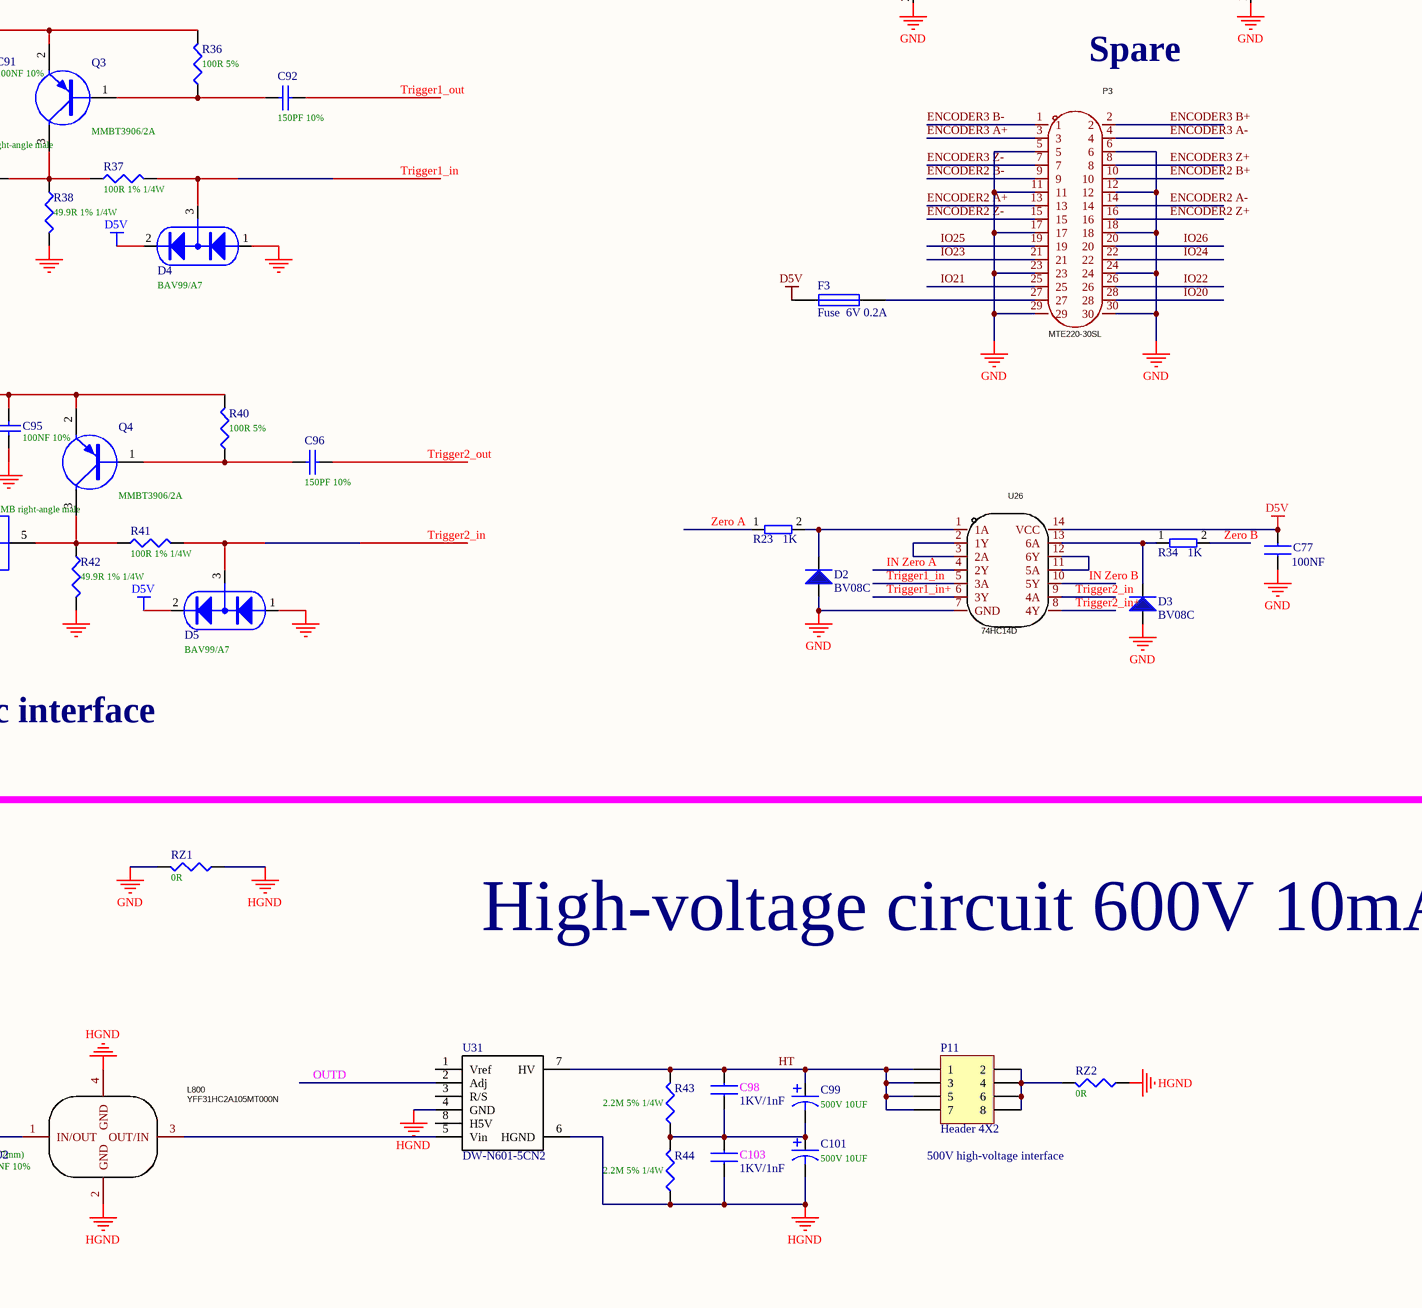
[diagram p0: MISC82191-3.SchDoc, bottom right]
# Altium project MISC82191-2.PrjPcb (part 2 of 4)

## Sheet MISC82191-3.SchDoc
size 965 x 596 mm

### Parts
C51  100NF 10%  [0805A]
C52  10pF/50V  [0603]
C53  10pF/50V  [0603]
C54  10pF/50V  [0603]
C55  10pF/50V  [0603]
C56  10pF/50V  [0603]
C57  10pF/50V  [0603]
C58  10pF/50V  [0603]
C59  10pF/50V  [0603]
C60  10pF/50V  [0603]
C61  100nF/50V  [0603]
C62  10pF/50V  [0603]
C63(NC)  10pF/50V  [0603]
C64  10pF/50V  [0603]
C65  10pF/50V  [0603]
C66  10pF/50V  [0603]
C67  10pF/50V  [0603]
C68（NC）  10pF/50V  [0603]
C69  100nF/50V  [0603]
C70  100nF/50V  [0603]
C71  100NF  [C0402]
C72  100NF  [C0402]
C73  100NF  [C0402]
C74  100NF  [C0402]
C75  100NF  [C0402]
C76  100NF  [C0402]
C77  100NF  [0603]
C78  100NF  [C0402]
C79  100NF  [C0402]
C80  100NF  [C0402]
C81  100NF  [C0402]
C82  100NF  [C0402]
C83  100NF  [C0402]
C85  100NF  [C0402]
C86  100NF  [C0402]
C87  100NF  [C0402]
C88  100NF  [C0402]
C89  100NF  [C0402]
C90  100NF  [C0402]
C91  100NF 10%  [0805R]
C92  150PF 10%  [0805R]
C95  100NF 10%  [0805R]
C96  150PF 10%  [0805R]
C97  10uF  25V 10%  [0805R]
C98  1KV/1nF  [3225[1210]]
C99  500V 10UF  [CAP-SMD_BD10.0-L10.3-W10.3-LS11.0-R-RD]
C100  220UF 25V (D6.3*7.7mm)  [CAP-SMD-6.3]
C101  500V 10UF  [CAP-SMD_BD10.0-L10.3-W10.3-LS11.0-R-RD]
C102  100NF 10%  [0805R]
C103  1KV/1nF  [3225[1210]]
C115  47uF 25V  [1206]
C116  47uF 25V  [1206]
C117  47uF 25V  [1206]
C501  100nF/50V  [0603]
C502  100nF/50V  [0603]
C704  10uF  25V 10%  [0805R]
C706  10uF  25V 10%  [0805R]
D2  BV08C  [SOD323]
D3  BV08C  [SOD323]
D4  BAV99/A7  [SOT-23]
D5  BAV99/A7  [SOT-23]
F1  Fuse  6V 0.2A  [0805]
F3  Fuse  6V 0.2A  [0805]
J1  0.8mm 2*50  [板对板座2*50]
J2  0.8mm 2*50  [板对板座2*50]
L11  600Ω-1.3A  [0805]
L12  600Ω-1.3A  [0805]
L13  600Ω-1.3A  [0805]
L14  600Ω-1.3A  [0805]
L15  600Ω-1.3A  [0805]
L16  600Ω-1.3A  [0805]
L17  600Ω-1.3A  [0805]
L18  600Ω-1.3A  [0805]
L19  600Ω-1.3A  [0805]
L20  XRCD54-4R7M(4.7uH 2A SMD,4.5x5.2mm)  [IND-SMD_L7.8-W7.0-A]
L80(NC)  600Ω-1.3A  [0805]
L104  YFF31HC2A105MT000N  [FILTER-SMD_4P-L3.2-W1.6-L_YFF31HC]
L105  YFF31HC2A105MT000N  [FILTER-SMD_4P-L3.2-W1.6-L_YFF31HC]
L106  YFF31HC2A105MT000N  [FILTER-SMD_4P-L3.2-W1.6-L_YFF31HC]
L800  YFF31HC2A105MT000N  [FILTER-SMD_4P-L3.2-W1.6-L_YFF31HC]
LED1  LED white body, red/green bicolour(Φ3/common anode) with 3mm single-hole square LED right-angle holder(7*6.4*7.4mm)  [DIP3B]
P2  Header 10  [2B-10]
P3  MTE220-30SL  [CONN-TH_MTE220-30SL]
P4  Header 20X2  [N0.8mm/40Pin-Plug]
P6  Header 20X2  [N0.8mm/40Pin-Plug]
P7  Header 7X2  [IDC-TH_14P-P2.54-V-R2-C7-S2.54]
P8  RF connector SMB-JWHD SMB right-angle male  [DIP-P]
P9  Header 20X2  [N0.8mm/40Pin-Plug]
P10  RF connector SMB-JWHD SMB right-angle male  [DIP-P]
P11  Header 4X2  [N0.8mm/8Pin-SOCKET]
P13  Header 20X2  [N0.8mm/40Pin-Plug]
P50  Analog output  [DIP-P]
P51  AD input  [DIP-P]
P52  gain  [DIP-P]
P53  (no value)  [DIP-P]
Q1  MMBT3904LT1(1AM)  [SOT23]
Q2  MMBT3904LT1(1AM)  [SOT23]
Q3  MMBT3906/2A  [SOT-23]
Q4  MMBT3906/2A  [SOT-23]
R19  100R 5%  [0603A]
R20  100R 5%  [0603A]
R23  1K  [0402]
R25  2K 5%  [0603A]
R26  2K 5%  [0603A]
R27  2K 5%  [0603A]
R28  2K 5%  [0603A]
R34  1K  [0402]
R35  100R 5%  [0805R]
R36  100R 5%  [0805R]
R37  100R 1% 1/4W  [AXIAL-0.45]
R38  49.9R 1% 1/4W  [AXIAL-0.5]
R39  100R 5%  [0805R]
R40  100R 5%  [0805R]
R41  100R 1% 1/4W  [AXIAL-0.45]
R42  49.9R 1% 1/4W  [AXIAL-0.5]
R43  2.2M 5% 1/4W  [AXIAL-0.5]
R44  2.2M 5% 1/4W  [AXIAL-0.5]
RJ1  HY911130A  [HY911130A]
RZ1  0R  [0805R]
RZ2  0R  [0805R]
U8  BV05C  [SOD-323]
U9  BV05C  [SOD-323]
U10  BV05C  [SOD-323]
U11  BV05C  [SOD-323]
U12  BV05C  [SOD-323]
U13  SMBJ33CA /33V  [DO-214AC(SMA)]
U14  BV05C  [SOD-323]
U15  BV05C  [SOD-323]
U16  BV05C  [SOD-323]
U17  AM26LV32EIPWR  [TSSOP-16_L5.0-W4.4-P0.65-LS6.4-BL]  (value not drawn)
U18  TXB0108RGYR  [QFN20]
U19  TXB0108RGYR  [QFN20]
U20  TXB0108RGYR  [QFN20]
U21  AM26LV32EIPWR  [TSSOP-16_L5.0-W4.4-P0.65-LS6.4-BL]  (value not drawn)
U22  AM26LV32EIPWR  [TSSOP-16_L5.0-W4.4-P0.65-LS6.4-BL]  (value not drawn)
U23  TXB0108RGYR  [QFN20]
U24  TXB0108RGYR  [QFN20]
U25  TXB0108RGYR  [QFN20]
U26  74HC14D  [SO-14]
U27  TXB0108RGYR  [QFN20]
U28  TXB0108RGYR  [QFN20]
U29  TXB0108RGYR  [QFN20]
U31  DW-N601-5CN2  [DW-N601-5CN2]
U501  74HC14D  [SO-14]
U707  74HC14D  [SO-14]

### Nets
3V3: C72.2 C74.2 C76.2 C79.2 C81.2 C83.2 C86.2 C90.2 LED1.2 P7.2 RJ1.11 RJ1.14 U18.2(VCCA) U18.10(OE) U19.2(VCCA) U19.10(OE) U20.2(VCCA) U20.10(OE) U23.2(VCCA) U23.10(OE) U24.2(VCCA) U24.10(OE) U25.2(VCCA) U25.10(OE) U27.2(VCCA) U27.10(OE) U29.2(VCCA) U29.10(OE)
13V: C115.1 C116.2 C117.2 J2.A1 J2.A2 J2.A3 J2.A4 J2.A5 J2.A6 J2.A7 J2.A8 J2.A9 J2.A10 J2.B1 J2.B2 J2.B3 J2.B4 J2.B5 J2.B6 J2.B7 J2.B8 J2.B9 J2.B10 L20.1 L106.3(OUT/IN)
-5.4V: L104.3(OUT/IN)
A6V: L105.3(OUT/IN)
A6V4: C706.2 L105.1(IN/OUT) P9.17 P9.18 P9.19 P9.20 P9.21 P9.22 P9.23 P9.24
D5V: C61.2 C69.2 C70.2 C71.1 C73.1 C75.1 C77.2 C78.1 C80.1 C82.1 C85.1 C87.1 C89.1 C501.2 C502.2 D4.2 D5.2 F1.2 F3.2 R35.2 R39.2 U17.4(G) U17.16(VCC) U18.19(VCCB) U19.19(VCCB) U20.19(VCCB) U21.4(G) U21.16(VCC) U22.4(G) U22.16(VCC) U23.19(VCCB) U24.19(VCCB) U25.19(VCCB) U26.14(VCC) U27.19(VCCB) U28.19(VCCB) U29.19(VCCB) U501.14(VCC) U707.14(VCC)
DGND: C54.2 C55.2 C59.2 C60.2 C61.1 C66.2 C67.1 C68（NC）.2 C69.1 C70.1 C71.2 C72.1 C73.2 C74.1 C75.2 C76.1 C77.1 C78.2 C79.1 C80.2 C81.1 C82.2 C83.1 C85.2 C86.1 C87.2 C88.1 C89.2 C90.1 C91.2 C95.2 C97.2 C115.2 C116.1 C117.1 C501.1 C502.1 C704.1 C706.1 D2.1 D3.1 D4.1 D5.1 J1.A2 J1.A5 J1.A8 J1.A11 J1.A14 J1.A17 J1.A20 J1.A23 J1.A25 J1.A28 J1.A31 J1.A34 J1.A37 J1.A40 J1.A42 J1.A45 J1.A48 J1.A50 J1.B2 J1.B5 J1.B8 J1.B11 J1.B14 J1.B17 J1.B20 J1.B23 J1.B25 J1.B28 J1.B31 J1.B34 J1.B37 J1.B40 J1.B42 J1.B45 J1.B48 J1.B50 J2.A11 J2.A12 J2.A13 J2.A14 J2.A15 J2.A16 J2.A17 J2.A18 J2.A19 J2.A20 J2.A23 J2.A26 J2.A29 J2.A32 J2.A35 J2.A38 J2.A41 J2.A44 J2.A47 J2.A50 J2.B11 J2.B12 J2.B13 J2.B14 J2.B15 J2.B16 J2.B17 J2.B18 J2.B19 J2.B20 J2.B21 J2.B22 J2.B23 J2.B24 J2.B26 J2.B29 J2.B32 J2.B35 J2.B38 J2.B41 J2.B44 J2.B47 J2.B50 L104.2(GND) L104.4(GND) L105.2(GND) L105.4(GND) L106.2(GND) L106.4(GND) P3.5 P3.6 P3.11 P3.12 P3.17 P3.18 P3.23 P3.24 P3.29 P3.30 P4.5 P4.6 P4.11 P4.12 P4.17 P4.18 P4.23 P4.24 P4.29 P4.30 P4.35 P4.36 P6.5 P6.6 P6.11 P6.12 P6.17 P6.18 P6.19 P6.23 P6.24 P6.29 P6.30 P6.35 P6.36 P7.3 P7.5 P7.7 P7.9 P7.11 P7.13 P8.1 P8.2 P8.3 P8.4 P9.11 P9.12 P9.13 P9.14 P9.15 P9.16 P9.25 P9.26 P9.27 P9.28 P9.29 P9.30 P10.1 P10.2 P10.3 P10.4 P13.9 P13.10 P13.11 P13.12 P13.17 P13.18 P13.23 P13.24 P13.25 P13.27 P13.29 P13.30 P13.31 P13.33 P13.35 P13.36 P13.37 P13.39 P50.1 P50.2 P50.3 P50.4 P51.1 P51.2 P51.3 P51.4 P52.1 P52.2 P52.3 P52.4 P53.1 P53.2 P53.3 P53.4 Q1.2(E) Q2.2(E) R27.1 R28.1 R38.1 R42.1 RZ1.2 U17.8(GND) U17.12(G#) U18.11(GND) U19.11(GND) U20.11(GND) U21.8(GND) U21.12(G#) U22.8(GND) U22.12(G#) U23.11(GND) U24.11(GND) U25.11(GND) U26.7(GND) U27.11(GND) U28.11(GND) U29.11(GND) U501.7(GND) U707.7(GND)  [also labelled GND]
HGND: C100.2 C101.2 C102.2 C103.2 L800.2(GND) L800.4(GND) R44.1 RZ1.1 RZ2.1 U31.4(GND) U31.6(HGND)
KGND: C51.2 C52.2 C53.2 C56.2 C57.2 C58.2 C62.1 C63(NC).1 C64.1 C65.1 P2.3 RJ1.10 RJ1.15(SH) RJ1.16(SH) U8.1 U9.1 U10.1 U11.1 U12.1 U13.2 U14.2 U15.2 U16.2
VCC1V8: C88.2 U28.2(VCCA) U28.10(OE)
1_A_N: C58.1 L14.2 P2.6 U12.2
1_A_P: C57.1 L13.2 P2.5 U11.2
1V8IO1: J1.A21
1V8IO2: J1.A22
1V8IO3: J1.A24
1V8IO4: J1.A27
1V8IO5: J1.A26
1V8IO6: J1.A29
1V8IO7: J1.A30
1V8IO8: J1.A32
1V8IO9: J1.A33
1V8IO10: J1.A35
1V8IO11: J1.A36
1V8IO12: J1.A38
1V8IO13: J1.A39
1V8IO14: J1.A41
1V8IO16: J1.A44
1V8IO17: J1.A46
1V8IO18: J1.A47
1V8IO19: P13.20 U28.1(A1)
1V8IO20: P13.22 U28.3(A2)
1V8IO21: P13.26 U28.4(A3)
1V8IO22: P13.28 U28.5(A4)
1V8IO23: P13.32 U28.6(A5)
1V8IO24: P13.34 U28.7(A6)
1V8IO25: P13.38 U28.8(A7)
1V8IO26: P13.40 U28.9(A8)
2_A_N: C65.2 L16.2 P2.8 U16.1
2_A_P: C52.1 L15.2 P2.7 U8.2
3_A_N: C63(NC).2 L18.2 L80(NC).2 P2.2 U14.1
3_A_P: C64.2 L17.2 P2.1 U15.1
3VIO23: J1.B19 U24.6(A5)
3VIO24: J1.B18 U24.5(A4)
3VIO25: J1.A18 U19.9(A8)
3VIO26: J1.B22 U24.8(A7)
3VIO27: J1.A4 U18.6(A5)
3VIO28: J1.B16 U19.8(A7)
3VIO29: J1.B15 U19.7(A6)
3VIO30: J1.B1 U18.5(A4)
3VIO31: J1.B3 U18.7(A6)
3VIO32: J1.A16 U19.6(A5)
3VIO33: J1.A15 U19.5(A4)
3VIO34: J1.B13 U19.3(A2)
3VIO40: J2.B27
3VIO41: J2.B28
3VIO42: J2.B30
3VIO43: J2.B25 U25.9(A8)
3VIO44: J2.B31 U25.4(A3)
3VIO45: J2.B33 U25.1(A1)
3VIO46: J2.B34 U20.8(A7)
3VIO47: J2.B36 U20.7(A6)
3VIO48: J2.B37 U20.6(A5)
3VIO49: J2.B39 U20.5(A4)
3VIO50: J2.B40 U20.4(A3)
3VIO51: J2.B42 U20.3(A2)
3VIO52: J2.B43 U20.1(A1)
3VIO53: J2.A27 U25.8(A7)
3VIO54: J2.A28 U25.7(A6)
3VIO55: J2.A30 U25.6(A5)
3VIO56: J2.A31 U25.5(A4)
3VIO57: J2.A33 U25.3(A2)
3VIO58: J2.A34 U20.9(A8)
3VIO60: J2.A37 U24.3(A2)
3VIO61: J2.A40 U19.4(A3)
3VIO62: J2.A39 U24.1(A1)
3VIO63: J2.A42
3VIO64: J2.A43
AK0: J2.A36 U24.4(A3)
AK1: P6.28 U27.12(B8)
AK2: P6.34 U27.13(B7)
AK3: P6.37 U27.17(B3)
AK4: P6.38 U27.14(B6)
AK5: P6.39 U27.16(B4)
AK6: P6.33 U27.18(B2)
AK7: P6.31 U27.20(B1)
AK8: P6.27 U29.12(B8)
AK9: P6.25 U29.13(B7)
AK10: P6.20 U29.17(B3)
AK11: U29.18(B2)
AK12: U29.15(B5)
AK13: P6.22 U29.16(B4)
AK16: U29.20(B1)
AS19: U24.13(B7)
AS20: P4.4 U18.15(B5)
AS23: P4.8 U18.16(B4)
AS24: P4.2 U18.14(B6)
AS27: P4.37 U19.18(B2)
AS28: P4.39 U19.17(B3)
Attn1: P4.33 U23.12(B8)
Attn2: P4.31 U23.13(B7)
Attn4: P4.27 U23.14(B6)
Attn8: P4.25 U23.15(B5)
Attn16: P4.21 U23.16(B4)
DAC Clk: J1.A7 P4.13
DAC Data: J1.B7 P4.15
DAC Strobe: J1.B6 P4.9
DATA_T: P6.40 U27.15(B5)
ENCODER2 A: U21.3(1Y) U501.13(6A)
ENCODER2 A+: P3.13 U21.2(1A)
ENCODER2 A-: P3.14 U21.1(1B)
ENCODER2 AA: U25.12(B8) U501.12(6Y)
ENCODER2 B: U21.5(2Y) U501.11(5A)
ENCODER2 B+: P3.10 U21.6(2A)
ENCODER2 B-: P3.9 U21.7(2B)
ENCODER2 BB: U25.13(B7) U501.10(5Y)
ENCODER2 Z: U21.11(3Y) U501.9(4A)
ENCODER2 Z+: P3.16 U21.10(3A)
ENCODER2 Z-: P3.15 U21.9(3B)
ENCODER2 ZZ: U25.14(B6) U501.8(4Y)
ENCODER3 A: U22.3(1Y) U25.17(B3)
ENCODER3 A+: P3.3 U22.2(1A)
ENCODER3 A-: P3.4 U22.1(1B)
ENCODER3 B: U22.5(2Y) U25.18(B2)
ENCODER3 B+: P3.2 U22.6(2A)
ENCODER3 B-: P3.1 U22.7(2B)
ENCODER3 Z: U22.11(3Y) U25.20(B1)
ENCODER3 Z+: P3.8 U22.10(3A)
ENCODER3 Z-: P3.7 U22.9(3B)
ENCODER A: U17.3(1Y) U501.1(1A)
ENCODER A_N: C55.1 L14.1 U17.1(1B)
ENCODER A_P: C54.1 L13.1 U17.2(1A)
ENCODER AA: U20.12(B8) U501.2(1Y)
ENCODER B: U17.5(2Y) U501.3(2A)
ENCODER B_N: C60.1 L16.1 U17.7(2B)
ENCODER B_P: C59.1 L15.1 U17.6(2A)
ENCODER BB: U20.13(B7) U501.4(2Y)
ENCODER Z: U17.11(3Y) U501.5(3A)
ENCODER Z_N: C68（NC）.1 L18.1 U17.9(3B)
ENCODER Z_P: C66.1 L17.1 U17.10(3A)
ENCODER ZZ: U20.14(B6) U501.6(3Y)
ETH_LED1: P13.16 RJ1.12
ETH_LED2: P13.14 RJ1.13
ETH_TD0_N: P13.6 RJ1.3
ETH_TD0_P: P13.8 RJ1.2
ETH_TD1_N: P13.2 RJ1.7
ETH_TD1_P: P13.4 RJ1.4
ETH_TD2_N: P13.5 RJ1.6
ETH_TD2_P: P13.7 RJ1.5
ETH_TD3_N: P13.1 RJ1.9
ETH_TD3_P: P13.3 RJ1.8
Gate/ON: U28.20(B1) U707.11(5A)
HP Filt En: P4.3 U18.12(B8)
HT: C98.1 C99.1 P11.1 P11.3 P11.5 P11.7 R43.2 U31.7(HV)
HV_SCL: J2.A46
HV_SDA: J2.A45
IN1: P4.19 U23.17(B3)
IN2: P4.7 U23.18(B2)
IN Zero A: U25.16(B4) U26.4(2Y)
IN Zero B: U25.15(B5) U26.10(5Y)
IO20: P3.28 U28.18(B2)
IO21: P3.25 U28.17(B3)
IO22: P3.26 U28.16(B4)
IO23: P3.21 U28.15(B5)
IO24: P3.22 U28.14(B6)
IO25: P3.19 U28.13(B7)
IO26: P3.20 U28.12(B8)
K0: P4.10 U24.17(B3)
K1: J1.B26 U27.9(A8)
K2: J1.B27 U27.8(A7)
K3: J1.B33 U27.4(A3)
K4: J1.B29 U27.7(A6)
K5: J1.B32 U27.5(A4)
K6: J1.B35 U27.3(A2)
K7: J1.B49 U27.1(A1)
K8: J1.B36 U29.9(A8)
K9: J1.B38 U29.8(A7)
K10: J1.B44 U29.4(A3)
K11: J1.B47 U29.3(A2)
K12: J1.B41 U29.6(A5)
K13: J1.B43 U29.5(A4)
K14: J1.B30 U27.6(A5)
K15: J1.B39
K16: J1.B46 U29.1(A1)
LB_A0: P4.28 U19.12(B8)
LB_A1: P4.26 U24.16(B4)
LB_A2: P4.22 U24.15(B5)
LB_A4: P4.20 U24.14(B6)
LB_A5: P4.16 U18.18(B2)
LB_A6: P4.14 U18.17(B3)
LED1: P13.19 R25.1
LED2: P13.21 R26.1
LP Filt En: P4.1 U18.13(B7)
OUTA: J2.B48
OUTB: J2.B49
OUTC: J2.A49
OUTD: J2.A48 U31.2(Adj)
S1: J1.A13 U23.9(A8)
S2: J1.B12 U23.8(A7)
S3: J1.A12 U23.7(A6)
S4: J1.B10 U23.6(A5)
S5: J1.B9 U23.5(A4)
S9: J1.A6 U18.9(A8)
S10: J1.B4 U18.8(A7)
S11: J1.A9 U23.3(A2)
S12: J1.A10 U23.4(A3)
S13: J1.A3 U18.4(A3)
S14: J1.A1 U18.3(A2)
S15: J1.B21 U24.7(A6)
T+: J2.B45 U29.7(A6)
T-: J2.B46
TCK: J2.A25 P7.6
TDI: J2.A21 P7.10
TDO: J2.A24 P7.8
TMS: J2.A22 P7.4
Trigger1_in: D4.3 R37.1 U26.5(3A)
Trigger1_in+: U20.18(B2) U26.6(3Y)
Trigger1_out: C92.1 U20.17(B3)
Trigger2_in: D5.3 R41.1 U26.9(4A)
Trigger2_in+: U20.16(B4) U26.8(4Y)
Trigger2_out: C96.1 U20.20(B1)
TT: P6.21 U29.14(B6)
U15_IN1: P4.40 U19.16(B4)
U15_IN2: P4.38 U19.15(B5)
U15_IN3: P4.34 U19.14(B6)
U15_IN4: P4.32 U19.13(B7)
UART_RXD: P13.13
UART_TXD: P13.15
Zero A: L12.1 R23.1
Zero B: L11.1 R34.2
NetC51_1: C51.1 RJ1.1
NetC53_1: C53.1 L11.2 P2.10 U9.2
NetC56_1: C56.1 L12.2 P2.9 U10.2
NetC62_2: C62.2 L19.2 P2.4 U13.1
NetC67_2: C67.2 F1.1 L19.1
NetC91_1: C91.1 Q3.2(E) R35.1 R36.1
NetC92_2: C92.2 Q3.1(B) R36.2
NetC95_1: C95.1 Q4.2(E) R39.1 R40.1
NetC96_2: C96.2 Q4.1(B) R40.2
NetC97_1: C97.1 L106.1(IN/OUT) P9.31 P9.32 P9.33 P9.34 P9.35 P9.36 P9.37 P9.38 P9.39 P9.40
NetC98_2: C98.2 C99.2 C101.1 C103.1 R43.1 R44.2
NetC100_1: C100.1 C102.1 L20.2 L800.1(IN/OUT)
NetC704_2: C704.2 L104.1(IN/OUT) P9.1 P9.2 P9.3 P9.4 P9.5 P9.6 P9.7 P9.8 P9.9 P9.10
NetD2_2: D2.2 R23.2 U26.1(1A)
NetD3_2: D3.2 R34.1 U26.13(6A)
NetF3_1: F3.1 P3.27
NetL80(NC)_1: L80(NC).1 U707.8(4Y)
NetL800_3: L800.3(OUT/IN) U31.5(Vin)
NetLED1_1: LED1.1 R20.2
NetLED1_3: LED1.3 R19.2
NetP8_5: P8.5 Q3.3(C) R37.2 R38.2
NetP10_5: P10.5 Q4.3(C) R41.2 R42.2
NetP11_2: P11.2 P11.4 P11.6 P11.8 RZ2.2
NetP50_5: P50.5 P51.5
NetP52_5: P52.5 P53.5
NetQ1_1: Q1.1(B) R26.2 R28.2
NetQ1_3: Q1.3(C) R20.1
NetQ2_1: Q2.1(B) R25.2 R27.2
NetQ2_3: Q2.3(C) R19.1
NetU26_2: U26.2(1Y) U26.3(2A)
NetU26_11: U26.11(5A) U26.12(6Y)
NetU707_9: U707.9(4A) U707.10(5Y)

Not connected (* = marked no-connect by the designer): J1 A19 A43 A49 B24; P6 1 2 3 4 7 8 9 10 13 14 15 16 26 32; P7 1 12 14; U17 13(4Y) 14(4A) 15(4B); U18 1(A1) 20(B1); U19 1(A1) 20(B1); U20 15(B5); U21 13(4Y) 14(4A) 15(4B); U22 13(4Y) 14(4A) 15(4B); U23 1(A1) 20(B1); U24 9(A8) 12(B8) 18(B2) 20(B1); U31 1(Vref) 3(R/S) 8(H5V); U707 1(1A) 2(1Y) 3(2A) 4(2Y) 5(3A) 6(3Y) 12(6Y) 13(6A)

### Layout directives
differential pair: ENCODER A_N, ENCODER A_P, ENCODER B_N, ENCODER B_P, ENCODER Z_N, ENCODER Z_P, ETH_TD0_N, ETH_TD0_P, ETH_TD1_N, ETH_TD1_P, ETH_TD2_N, ETH_TD2_P, ETH_TD3_N, ETH_TD3_P

### Notes on the sheet
- Encoder uses PNP, incremental, step/direction
- Encoder: O V V V 6 - 1 0 -  2 D
- MINI miniature rotary encoder, quadrature/step-direction incremental, smart car pulse angle sensor
- Transmit interface
- Encoder interface
- Output 2S high level as switch signal
- Receive interface
- Status LED
- Spare
- Core board debug connector
- P8\P10 sync interface
- High-voltage circuit 600V 10mA output
- (near P11) 500V high-voltage interface
- Core board connector
- PS Ethernet

### Library data of the parts
C51 C91 C92 C95-C97 C102 C115-C117 C704 C706 = CAP: Capacitor
C52-C62 C63(NC) C64-C67 C68（NC） C69 C70 C501 C502 = CAP: CC-50V-106-±10%-[1206]
C71-C83 C85-C90 C98 C103 = CAP
C99 C101 = CAPACITOR
C100 = CAPACITOR_1: Capacitor
D2 D3 = D
D4 D5 = D1: Diode
F1 F3 = Fuse 1: Fuse
L11-L19 L80(NC) = L: BLM18KG601SN-[0603]/Murata
L20 = L
L104-L106 L800 = YFF31HC2A105MT000N: Manufacturer: TDK; Add into BOM: yes; Nominal Capacitance: 1uF; CapacitanceTolerance: ±20%; DC Rated Voltage: 100V; Rated Current: 6A; DC Resistance: 5mΩ; Name: YFF31HC2A105MT000N; Symbol: YFF31HC2A105MT000N; Device: YFF31HC2A105MT000N; LCSC Part Name: 1uF(105) ±20% 100V; Supplier Part: C113216; Manufacturer Part: YFF31HC2A105MT000N; Supplier Footprint: SMD-4P,1.6x3.2mm; JLCPCB Part Class: Extended Part; Datasheet: https://atta.szlcsc.com/upload/public/pdf/source/20180326/C113216_F6F81E50B9805DA3D7C436129903DEBD.pdf; Supplier: LCSC; Convert to PCB: yes; Operating Temperature: -55℃~+125℃
LED1 = LED_2
P2 = Header 10: Header, 10-Pin; LatestRevisionDate: 17-Jul-2002; LatestRevisionNote: Re-released for DXP Platform.; Publisher: Altium Limited
P3 = MTE220-30SL: Manufacturer: MINTRON(明硕); Add into BOM: yes; Connector Type: Box header latch; Pitch: 2mm; Structure: 2x15P; Holder Type: Through-hole; Pin Number in each Row: 15; Symbol: MTE220-30SL; Device: MTE220-30SL; LCSC Part Name: 2mm 2x15P 排数:2 每排P数:15; Supplier Part: C713798; Manufacturer Part: MTE220-30SL; Supplier Footprint: 插件,P=2mm; JLCPCB Part Class: Extended Part; Datasheet: https://atta.szlcsc.com/upload/public/pdf/source/20200731/C713794_07CB2E9D8B2AEEC374D2510E201C2D81.pdf; Supplier: LCSC; Convert to PCB: yes; Row Spacing: 2mm; Number of Rows: 2; Contact Material: Brass; Contact Plating: -
P4 P6 P9 P13 = Header 20X2: Header, 20-Pin, Dual row; LatestRevisionDate: 17-Jul-2002; LatestRevisionNote: Re-released for DXP Platform.; Publisher: Altium Limited
P7 = Header 7X2: Header, 7-Pin, Dual row; LatestRevisionDate: 17-Jul-2002; LatestRevisionNote: Re-released for DXP Platform.; Publisher: Altium Limited
P8 P10 P50-P53 = JA1
P11 = Header 4X2: Header, 4-Pin, Dual row; LatestRevisionDate: 17-Jul-2002; LatestRevisionNote: Re-released for DXP Platform.; Publisher: Altium Limited
Q1 Q2 = NPN: NPN Transistor
Q3 Q4 = PNP: PNP Transistor
R19 R20 R25-R28 R35-R44 RZ1 RZ2 = RES1
R23 R34 = RES
U8-U12 U14-U16 = SMAJ18CA 18V: BV05C-[SOD-323]/Bencent
U13 = SMAJ18CA 18V
U17 U21 U22 = AM26LV32EIPWR: Manufacturer: TI(德州仪器); Add into BOM: yes; Symbol: AM26LV32EIPWR; Device: AM26LV32EIPWR; LCSC Part Name: AM26LV32EIPWR; Supplier Part: C404024; Manufacturer Part: AM26LV32EIPWR; Supplier Footprint: TSSOP-16; JLCPCB Part Class: Extended Part; Datasheet: https://www.ti.com/cn/lit/gpn/am26lv32e; Supplier: LCSC; Convert to PCB: yes; Comment_1: AM26LV32EIPWR
U26 U501 U707 = 74HC14D,653: Manufacturer: Nexperia(安世); Add into BOM: yes; Input Type: Schmitt trigger; Supply Voltage(Single): 2V~6V; Supply Current (Max): 2uA; Number of Circuits: 6; Number of Inputs: 1; Sink Current: 5.2mA; High level range (VIH): 1.5V~4.2V; Low level range (VIL): 300mV~1.2V; Max Propagation Delay: 21ns@6V,50pF; Symbol: 74HC14D,653; Device: 74HC14D,653; LCSC Part Name: 六路施密特触发反相器; Supplier Part: C5605; Manufacturer Part: 74HC14D,653; Supplier Footprint: SOIC-14; JLCPCB Part Class: Basic Part; Datasheet: https://atta.szlcsc.com/upload/public/pdf/source/20170209/1486607341486.pdf; Supplier: LCSC; Convert to PCB: yes; Source Current: 5.2mA; Series: 74HC series; Operating Temperature: -40℃~+125℃; Comment_1: 74HC14D,653

## Sheet MISC82191-5.SchDoc
size OrCAD E
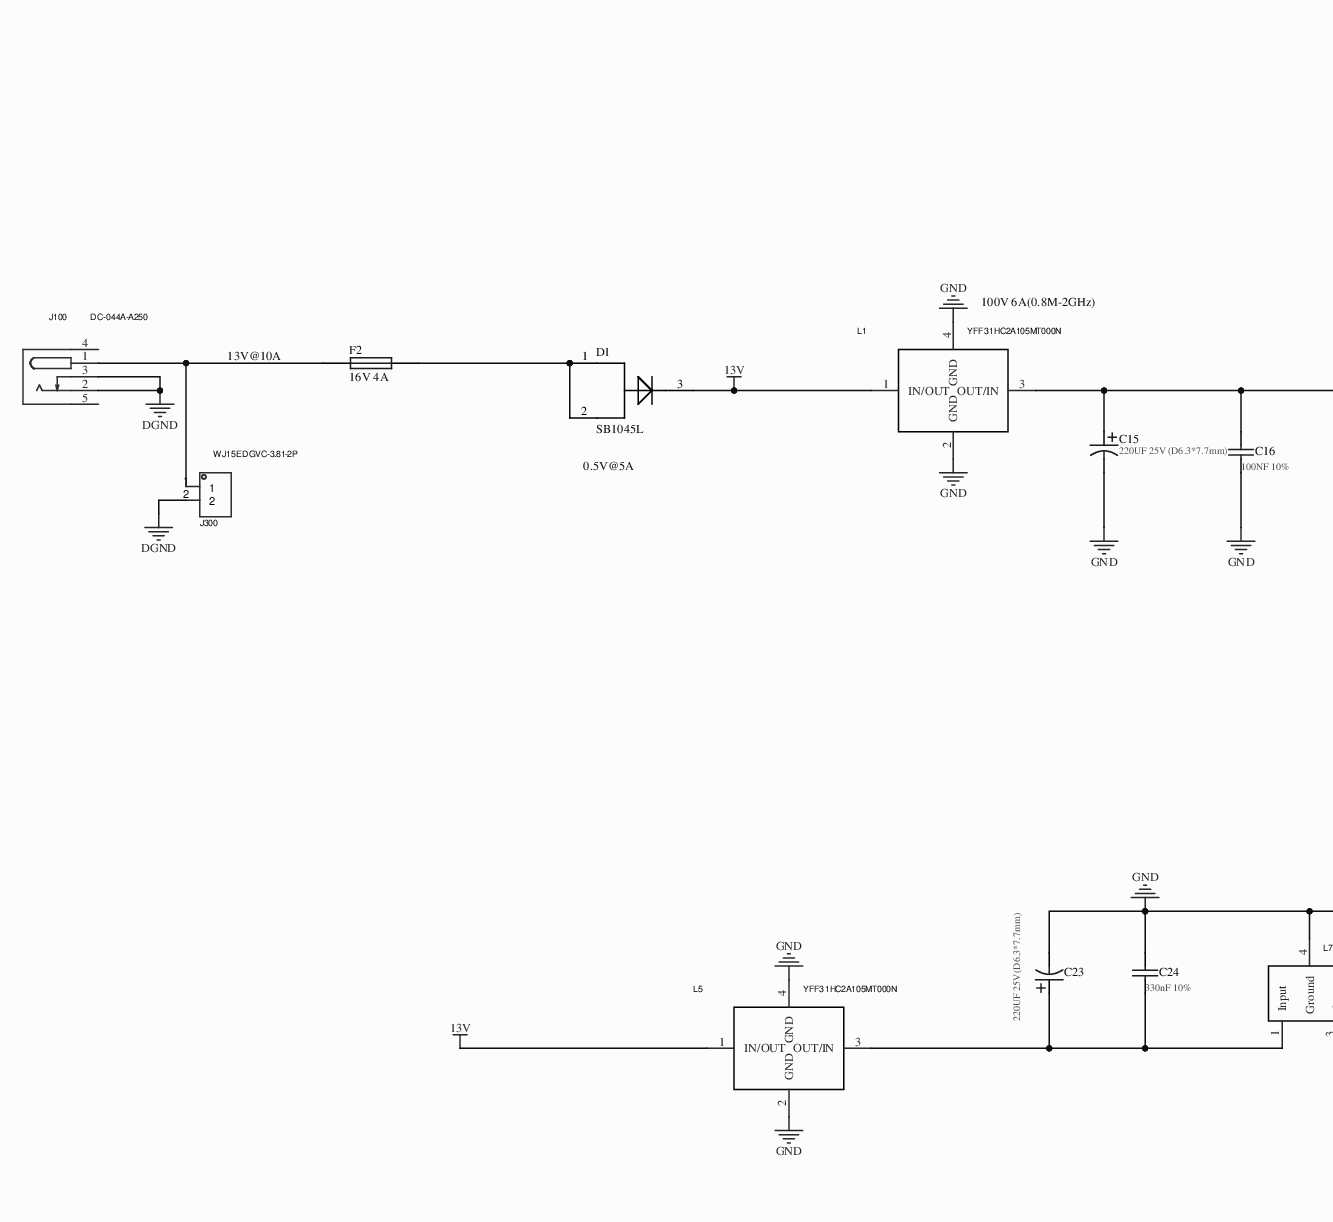
[diagram p1: MISC82191-5.SchDoc, top left]
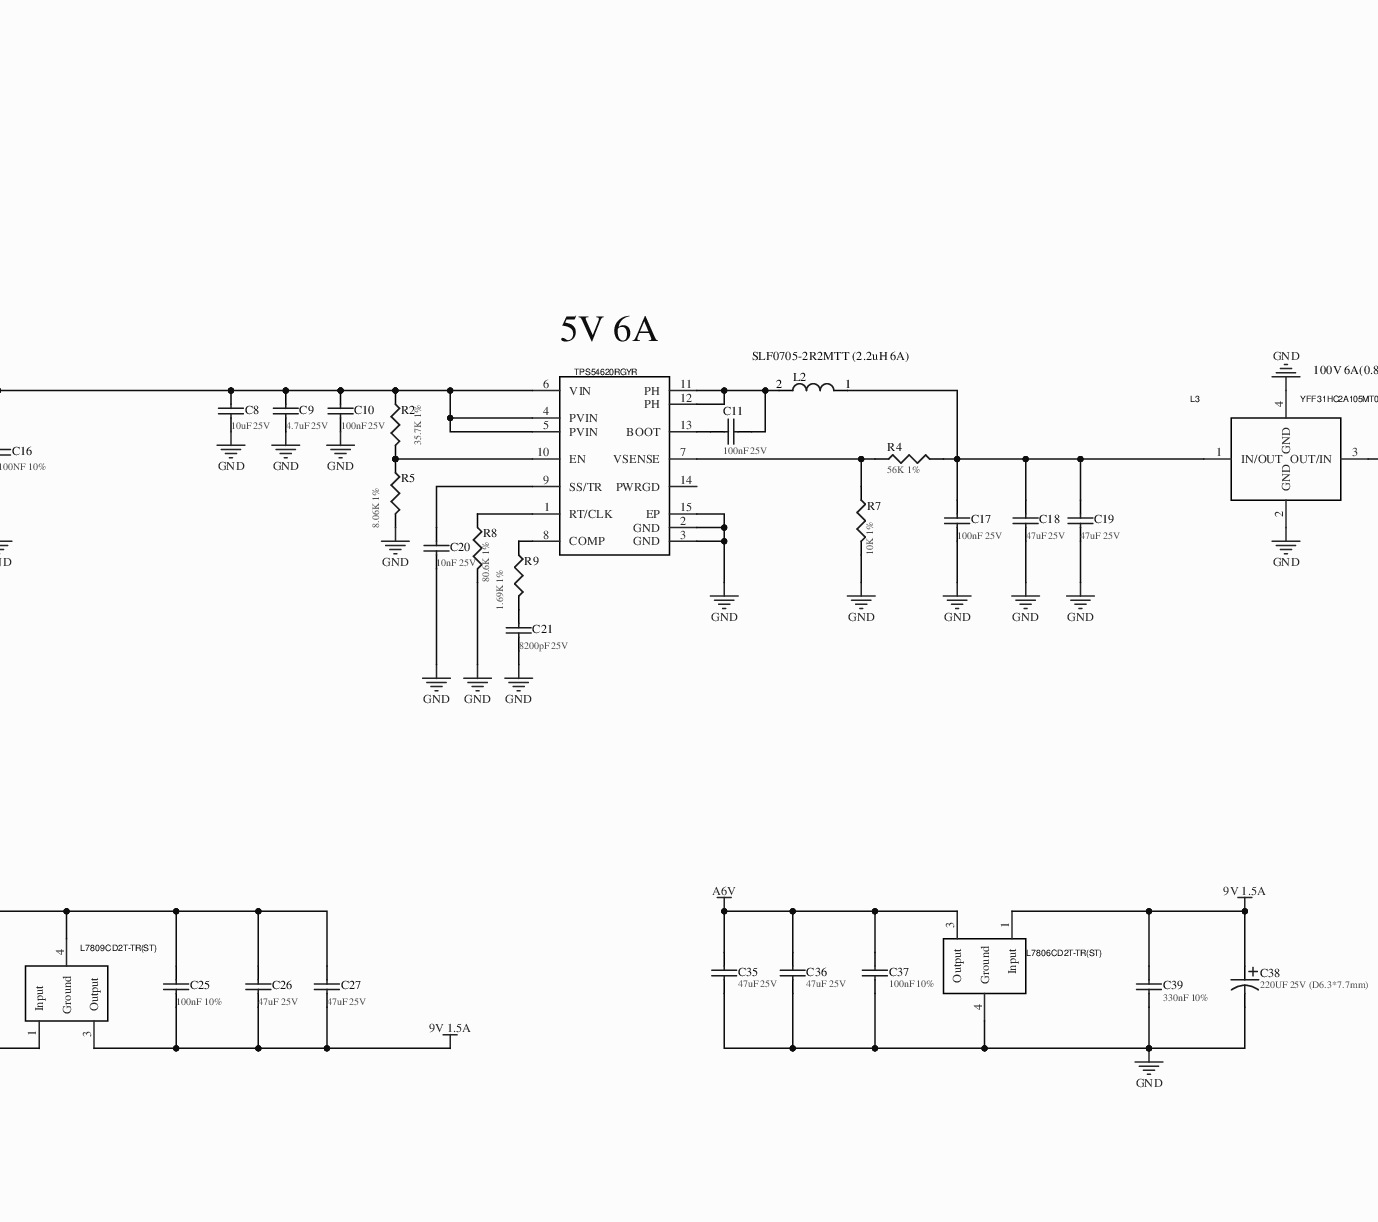
[diagram p2: MISC82191-5.SchDoc, top middle]
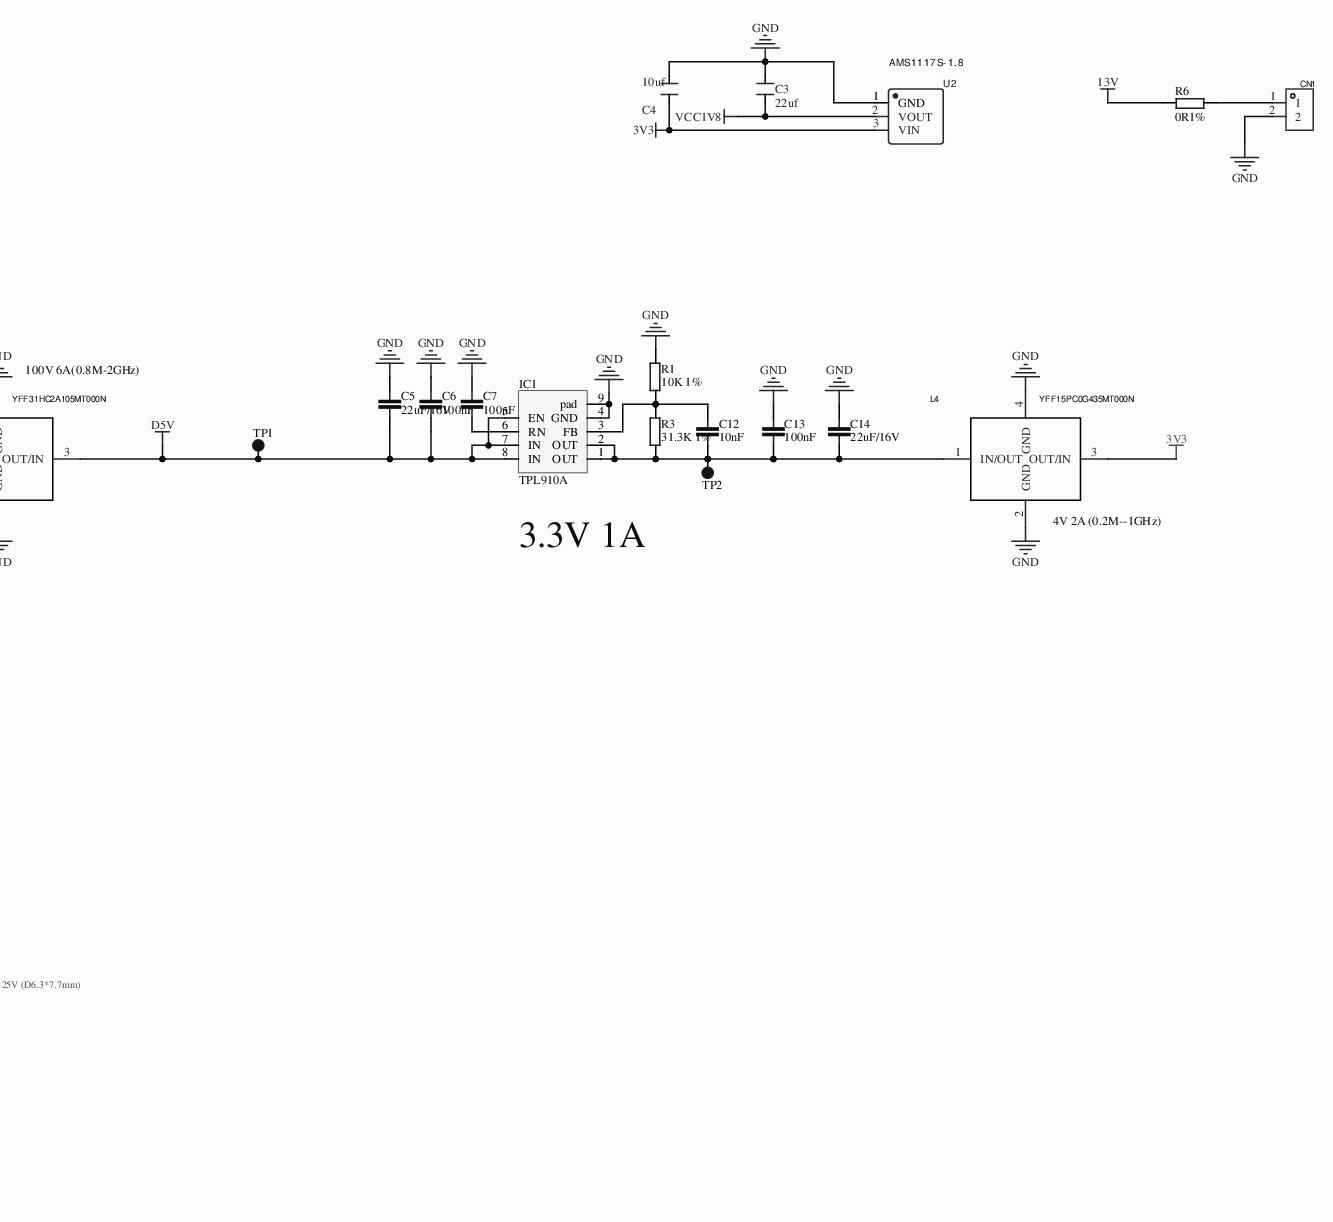
[diagram p3: MISC82191-5.SchDoc, top right]
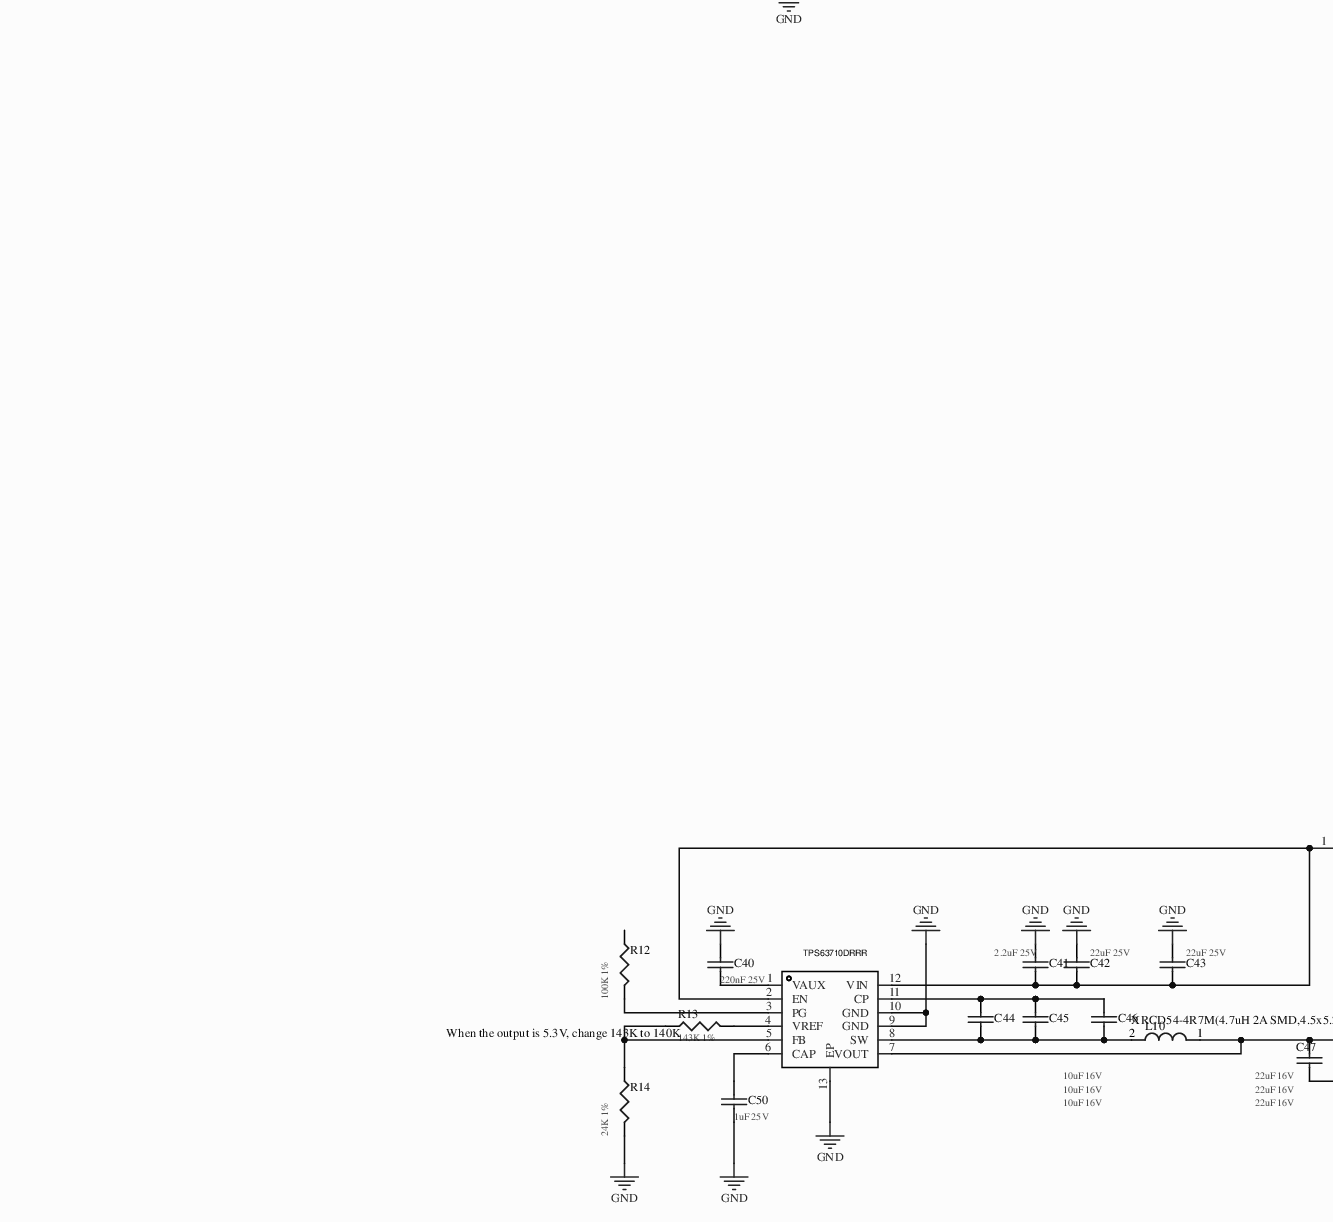
[diagram p4: MISC82191-5.SchDoc, bottom left]
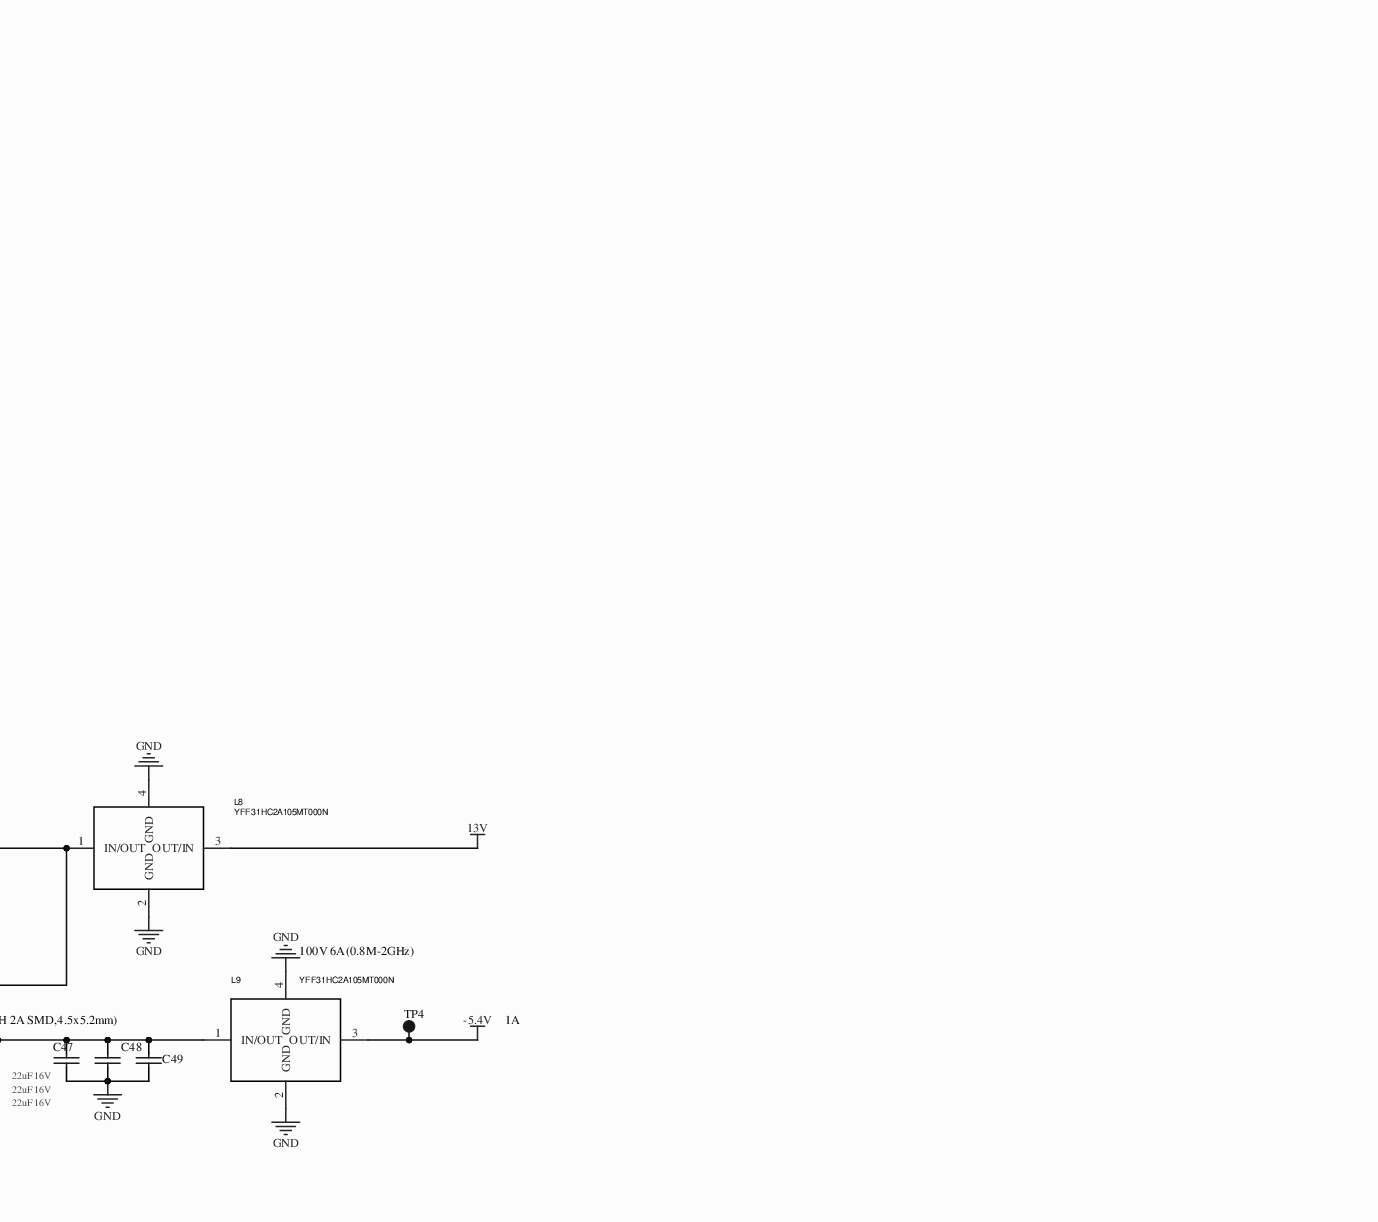
[diagram p5: MISC82191-5.SchDoc, bottom middle]

### Parts
C3  22uf  [1206]